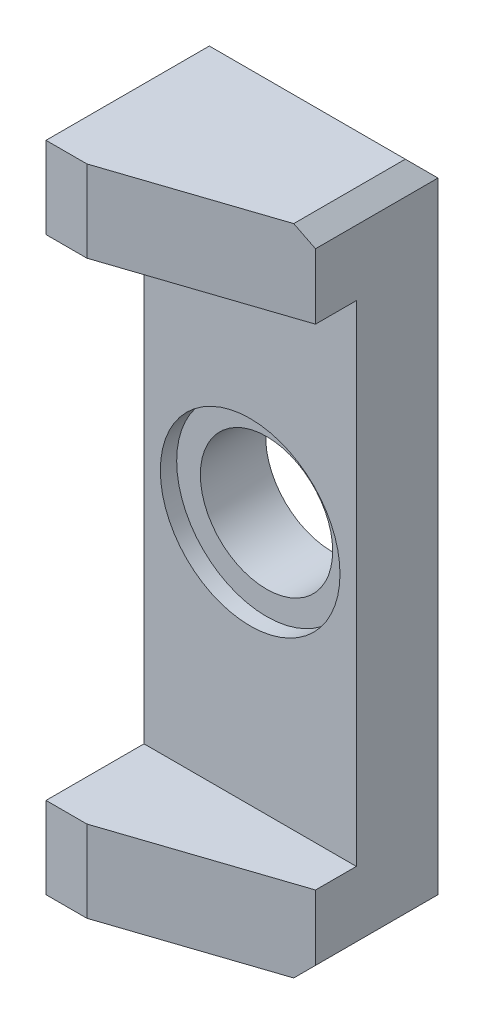
from build123d import *

# Parameters (mm, degrees)
SKETCH_1_W             = 26
SKETCH_1_H             = 80
EXTRUDE_1_DEPTH        = 10
SKETCH_2_R             = 8.1
CUT_EXTRUDE_1_DEPTH    = 44.231932642
EXTRUDE_2_DEPTH        = 10
CHAMFER_1_SIZE         = 2
CHAMFER_2_SIZE         = 2
SKETCH_9_R             = 11
CUT_EXTRUDE_2_DEPTH    = 2
HOLE_WIZARD_M4_1_D     = 3.3
HOLE_WIZARD_M4_1_DEPTH = 10.1
HOLE_WIZARD_M4_1_TIP   = 0.991420021


with BuildPart() as part:
    # 草图1 → 凸台-拉伸1 (new body)
    with BuildSketch(Plane.XY):
        Rectangle(SKETCH_1_W, SKETCH_1_H)
    extrude(amount=EXTRUDE_1_DEPTH)

    # 草图2 → 切除-拉伸1 (cut, through all)
    with BuildSketch(Plane.XY.offset(10)):
        Circle(SKETCH_2_R)
    extrude(amount=-CUT_EXTRUDE_1_DEPTH, mode=Mode.SUBTRACT)

    # 草图7 → 凸台-拉伸2 (add)
    with BuildSketch(Plane(origin=(0, 40, 0), x_dir=(1, 0, 0), z_dir=(0, 1, 0))):
        Polygon((13, -10), (13, -15), (-8, -22), (-13, -22), (-13, -10), align=None)
    extrude_2 = extrude(amount=-EXTRUDE_2_DEPTH)

    # 镜向1: 凸台-拉伸2 across plane
    add(extrude_2.mirror(Plane.ZX))

    # 倒角1
    chamfer_1_edges = [part.edges().sort_by_distance(p)[0] for p in [
        (13, -40, 7.5),
        (13, 40, 7.5),
    ]]
    chamfer(chamfer_1_edges, length=CHAMFER_1_SIZE)

    # 倒角2
    chamfer_2_edges = [part.edges().sort_by_distance(p)[0] for p in [
        (-1, -40, 0),
        (-1, 40, 0),
    ]]
    chamfer(chamfer_2_edges, length=CHAMFER_2_SIZE)

    # 草图9 → 切除-拉伸2 (cut)
    with BuildSketch(Plane(origin=(0, 0, 10), x_dir=(-1, 0, 0), z_dir=(0, 0, -1))):
        Circle(SKETCH_9_R)
    extrude(amount=CUT_EXTRUDE_2_DEPTH, mode=Mode.SUBTRACT)

    # M4 螺纹孔1
    with Locations(Plane.ZY.offset(13)):
        with Locations((17, 35), (7, 35), (7, -35), (17, -35)):
            Hole(HOLE_WIZARD_M4_1_D / 2, depth=HOLE_WIZARD_M4_1_DEPTH)
            with Locations((0, 0, -(HOLE_WIZARD_M4_1_DEPTH + HOLE_WIZARD_M4_1_TIP / 2))):  # 118° drill point
                Cone(0, HOLE_WIZARD_M4_1_D / 2, HOLE_WIZARD_M4_1_TIP, mode=Mode.SUBTRACT)


solid = part.part
